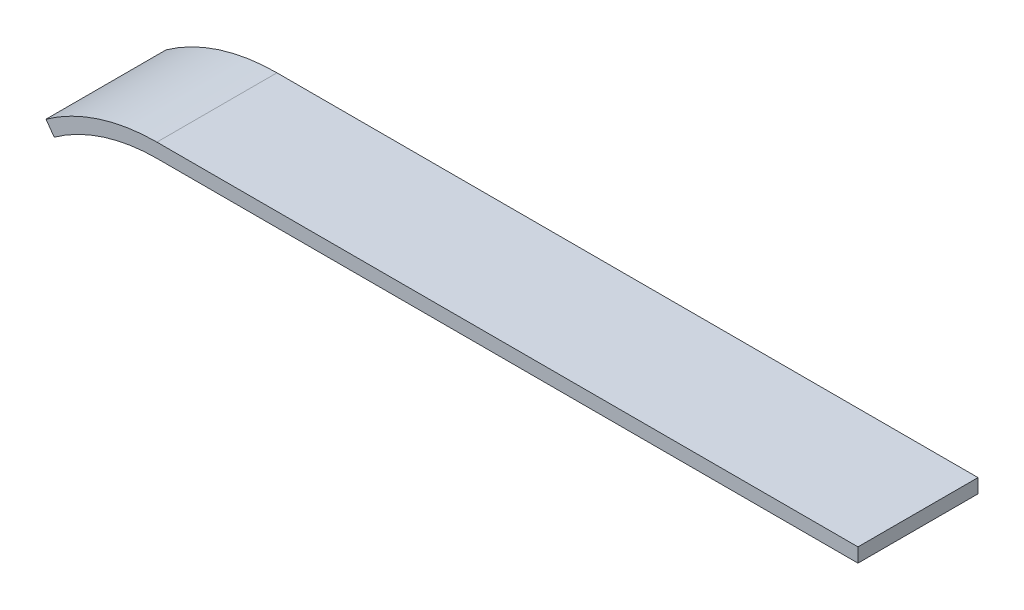
SolidWorks part; units mm, degrees
material "普通碳钢"
ref_plane "Front Plane" through (0, 0, 0) normal (0, 0, 1) x (1, 0, 0)
ref_plane "Top Plane" through (0, 0, 0) normal (0, 1, 0) x (1, 0, 0)
ref_plane "Right Plane" through (0, 0, 0) normal (1, 0, 0) x (0, 0, -1)
sketch "Sketch1" plane through (0, 0, 0) normal (0, 0, 1) x (1, 0, 0)
  line L0 (0, 0) -> (-595.7487, 0)
  line L1 (55, 0) -> (-55, 0) construction
  line L2 (0, -12) -> (-595.7487, -12)
  line L3 (-683.0184, -40) -> (-690, -30.24)
  line L4 (0, 0) -> (0, -12)
  line L5 (0, -55) -> (0, 55) construction
  line L6 (0, -12) -> (-595.7487, -12) construction
  arc A0 (-595.7487, 0) -> (-690, -30.24) centre (-595.7487, -162) ccw
  arc A1 (-595.7487, -12) -> (-683.0184, -40) centre (-595.7487, -162) ccw
  dimension "D3" = 150
  dimension "D4" = 690
  dimension "D5" = 40
  dimension "D1" = 12
extrude "Boss-Extrude1" add sketch "Sketch1" along normal blind 102
